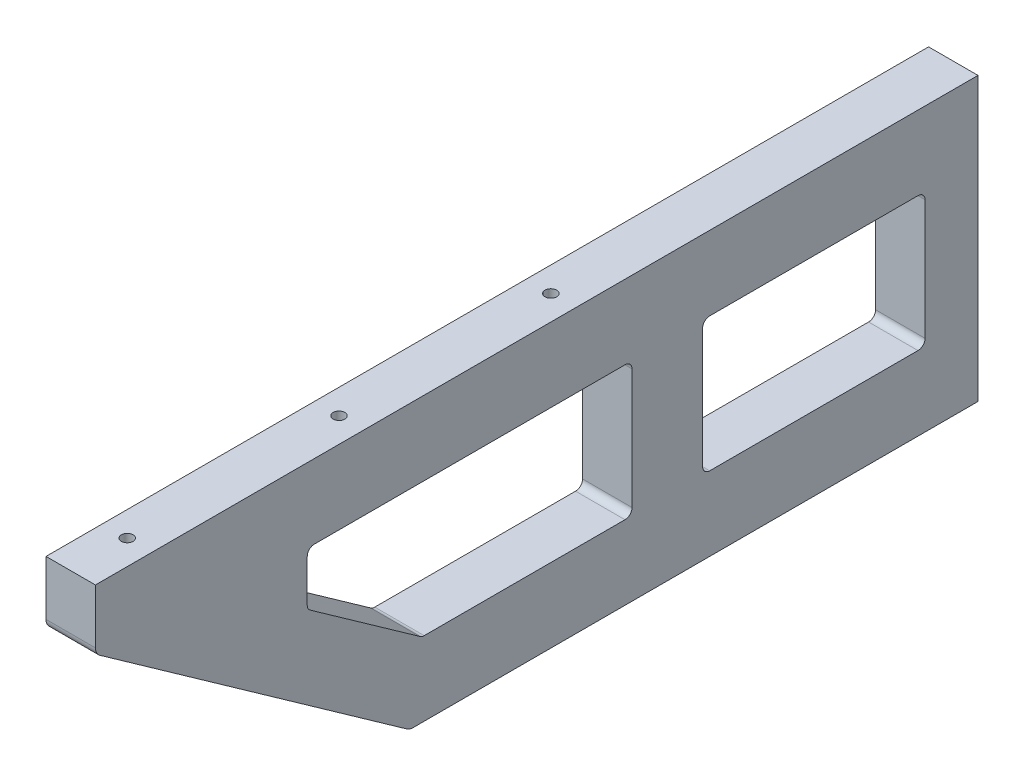
SolidWorks part; units mm, degrees
ref_plane "Front Plane" through (0, 0, 0) normal (0, 0, 1) x (1, 0, 0)
ref_plane "Top Plane" through (0, 0, 0) normal (0, 1, 0) x (1, 0, 0)
ref_plane "Right Plane" through (0, 0, 0) normal (1, 0, 0) x (0, 0, -1)
other "Configuration Table"
sketch "Sketch3" plane through (50, 414.5474, -101) normal (-1, 0, 0) x (0, 0, -1)
  line L0 (-101, 210.8045) -> (-101, 290.8045)
  line L6 (-101, 290.8045) -> (-262, 290.8045)
  line L9 (-351, 210.8045) -> (-101, 210.8045)
  line L10 (-262, 290.8045) -> (-351, 227.8045)
  line L11 (-351, 227.8045) -> (-351, 210.8045)
  dimension "D1" = 80
  dimension "D2" = 250
  dimension "D3" = 161
  dimension "D4" = 17
extrude "Boss-Extrude1" add sketch "Sketch3" along normal mid plane 14
sketch "Sketch4" plane through (57, 0, 0) normal (1, 0, 0) x (0, 0, -1)
  line L0 (0, 163.7429) -> (-15, 163.7429) construction
  line L1 (-15, 182.7429) -> (-78, 182.7429)
  line L2 (-15, 182.7429) -> (-15, 144.7429)
  line L3 (-15, 144.7429) -> (-78, 144.7429)
  line L4 (-78, 182.7429) -> (-78, 144.7429)
  line L5 (0, 203.7429) -> (0, 123.7429) construction
  dimension "D1" = 63
  dimension "D2" = 38
  dimension "D3" = 15
extrude "Cut-Extrude1" cut sketch "Sketch4" against normal through all
fillet "Fillet1" radius 2 4 edges at (50, 144.7429, 78) (50, 144.7429, 15) (50, 182.7429, 15) (50, 182.7429, 78)
sketch "Sketch5" plane through (57, 0, 0) normal (1, 0, 0) x (0, 0, -1)
  line L0 (-76, 144.7429) -> (-17, 144.7429) construction
  line L1 (-98, 144.7429) -> (-157.5079, 144.7429)
  line L2 (-98, 144.7429) -> (-98, 182.7429)
  line L3 (-98, 182.7429) -> (-190, 182.7429)
  line L5 (-17, 182.7429) -> (-76, 182.7429) construction
  line L6 (-78, 180.7429) -> (-78, 146.7429) construction
  line L7 (-157.5079, 144.7429) -> (-190, 167.7429)
  line L8 (-190, 167.7429) -> (-190, 182.7429)
  line L9 (-161, 123.7429) -> (-250, 186.7429) construction
  line L10 (-250, 186.7429) -> (-250, 203.7429) construction
  dimension "D1" = 20
  dimension "D2" = 15
  dimension "D3" = 60
extrude "Cut-Extrude2" cut sketch "Sketch5" against normal through all
fillet "Fillet2" radius 2 5 edges at (50, 144.7429, 157.5079) (50, 167.7429, 190) (50, 182.7429, 190) (50, 182.7429, 98) (50, 144.7429, 98)
hole_wizard "M5 Tapped Hole1" positions "Sketch6" profile "Sketch7" tap size "M5" standard "GB"
sketch "Sketch6" plane through (0, 0, 0) normal (0, 0, -1) x (-1, 0, 0)
  point P0 (-50.5, 188.7429)
  point P3 (-50, 138.7454)
cosmetic thread "HoleThreadLine1" parameters "D1"=10, "D2"=5
cosmetic thread "HoleThreadLine2" parameters "D1"=10, "D2"=5
sketch "Sketch7" plane through (50.5, 188.7429, 0) normal (1, 0, 0) x (0, 1, 0)
  line L0 (0, 0) -> (0, 15.2618)
  line L1 (0, 15.2618) -> (2.1, 14)
  line L2 (2.1, 14) -> (2.1, 0)
  line L5 (2.1, 0) -> (0, 0)
  line L10 (0, 15.2618) -> (-2.1, 14) construction
  line L11 (0, -6.35) -> (0, 107.95) construction
  dimension "螺纹孔钻头直径" = 4.2
  dimension "螺纹孔钻头深度" = 14
  dimension "导头角度" = 118
hole_wizard "M4 Tapped Hole1" positions "Sketch8" profile "Sketch9" tap size "M4" standard "GB"
sketch "Sketch8" plane through (0, 203.7429, 0) normal (0, 1, 0) x (1, 0, 0)
  point P0 (50, -114)
  point P3 (50, -174)
  point P6 (50, -234)
sketch "Sketch9" plane through (50, 203.7429, 114) normal (1, 0, 0) x (0, 0, 1)
  line L0 (0, 0) -> (0, 12.4914)
  line L1 (0, 12.4914) -> (1.65, 11.5)
  line L2 (1.65, 11.5) -> (1.65, 0)
  line L5 (1.65, 0) -> (0, 0)
  line L10 (0, 12.4914) -> (-1.65, 11.5) construction
  line L11 (0, -6.35) -> (0, 107.95) construction
  dimension "螺纹孔钻头直径" = 3.3
  dimension "螺纹孔钻头深度" = 11.5
  dimension "导头角度" = 118
cosmetic thread "HoleThreadLine3" parameters "D1"=8, "D2"=4
cosmetic thread "HoleThreadLine4" parameters "D1"=8, "D2"=4
cosmetic thread "HoleThreadLine5" parameters "D1"=8, "D2"=4
fillet "Fillet3" radius 3 2 edges at (50, 123.7429, 161) (50, 186.7429, 250)
